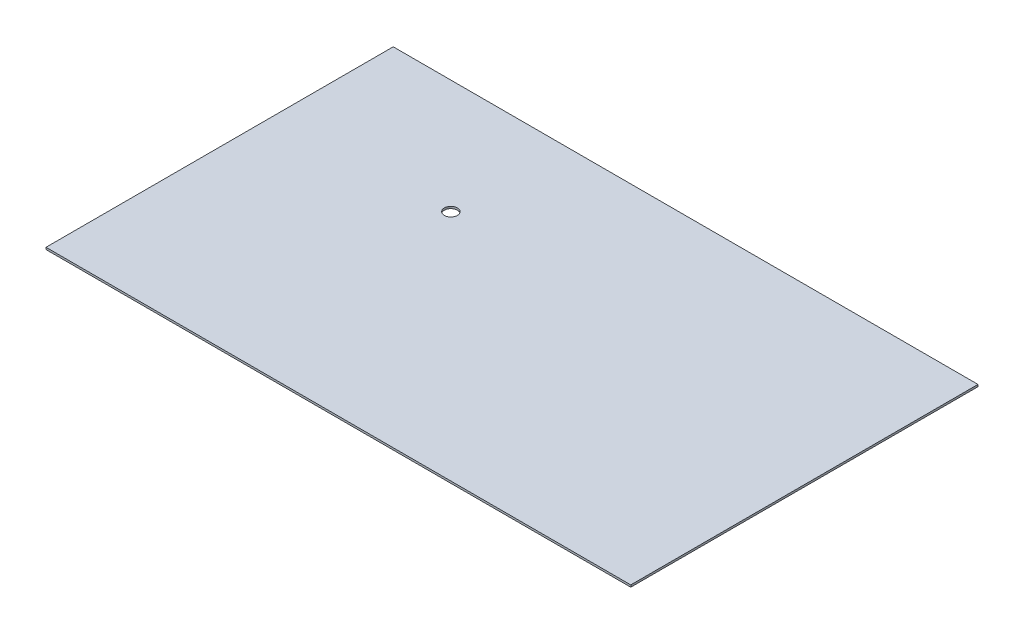
SolidWorks part; units mm, degrees
material "A3"
ref_plane "前视基准面" through (0, 0, 0) normal (0, 0, 1) x (1, 0, 0)
ref_plane "上视基准面" through (0, 0, 0) normal (0, 1, 0) x (1, 0, 0)
ref_plane "右视基准面" through (0, 0, 0) normal (1, 0, 0) x (0, 0, -1)
sketch "草图1" plane through (0, 0, 0) normal (0, 1, 0) x (1, 0, 0)
  line L0 (-235, 690) -> (-235, -690) construction
  line L1 (-1162, -690) -> (1162, -690)
  line L2 (-1162, -690) -> (-1162, 690)
  line L3 (-1162, 690) -> (1162, 690)
  line L4 (1162, -690) -> (1162, 690)
  line L5 (-1162, -690) -> (1162, 690) construction
  line L6 (-1162, 690) -> (1162, -690) construction
  line L7 (0, 690) -> (0, 0) construction
  line L8 (116.05, 672) -> (-116.05, 672) construction
  line L9 (-1162, 530) -> (1162, 530) construction
  line L10 (-1162, 360) -> (1162, 360) construction
  line L11 (-1162, 172) -> (1162, 172) construction
  line L12 (1170, -698) -> (-1170, -698) construction
  circle A2 centre (-480, 237) radius 26
  point P0 (0, 0)
  dimension "D6" = 18
  dimension "D8" = 235
  dimension "D9" = 52
  dimension "D11" = 480
  dimension "D7" = 927
  dimension "D10" = 8
  dimension "D1" = 1380
  dimension "D2" = 2324
  dimension "D3" = 160
  dimension "D4" = 330
  dimension "D5" = 188
extrude "凸台-拉伸1" add sketch "草图1" along normal mid plane 8
